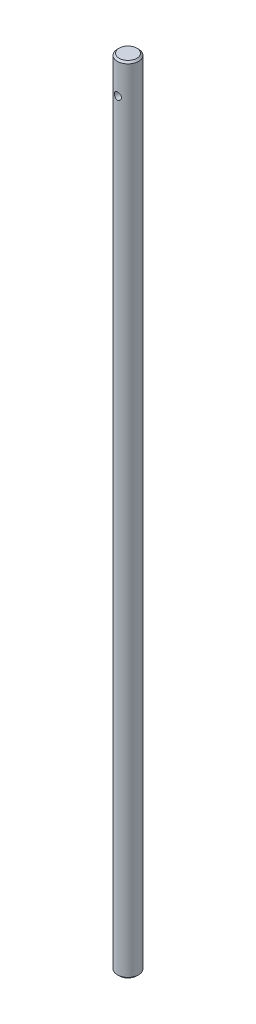
SolidWorks part; units mm, degrees
material "1060 Alloy"
ref_plane "Front Plane" through (0, 0, 0) normal (0, 0, 1) x (1, 0, 0)
ref_plane "Top Plane" through (0, 0, 0) normal (0, 1, 0) x (1, 0, 0)
ref_plane "Right Plane" through (0, 0, 0) normal (1, 0, 0) x (0, 0, -1)
other "mo"
sketch "Sketch1" plane through (0, 0, 0) normal (0, 1, 0) x (1, 0, 0)
  circle A0 centre (0, 0) radius 6
  dimension "D1" = 12
extrude "Boss-Extrude1" add sketch "Sketch1" along normal mid plane 450
chamfer "Chamfer1" distance 1 angle 45 2 edges at (0, -225, 6) (0, 225, 6)
sketch "Sketch2" plane through (0, 0, 0) normal (0, 0, 1) x (1, 0, 0)
  line L0 (5, 225) -> (-5, 225) construction
  circle A0 centre (0, 207) radius 2
  dimension "D1" = 18
  dimension "D2" = 4
extrude "Cut-Extrude1" cut sketch "Sketch2" against normal through all and the other way through all
